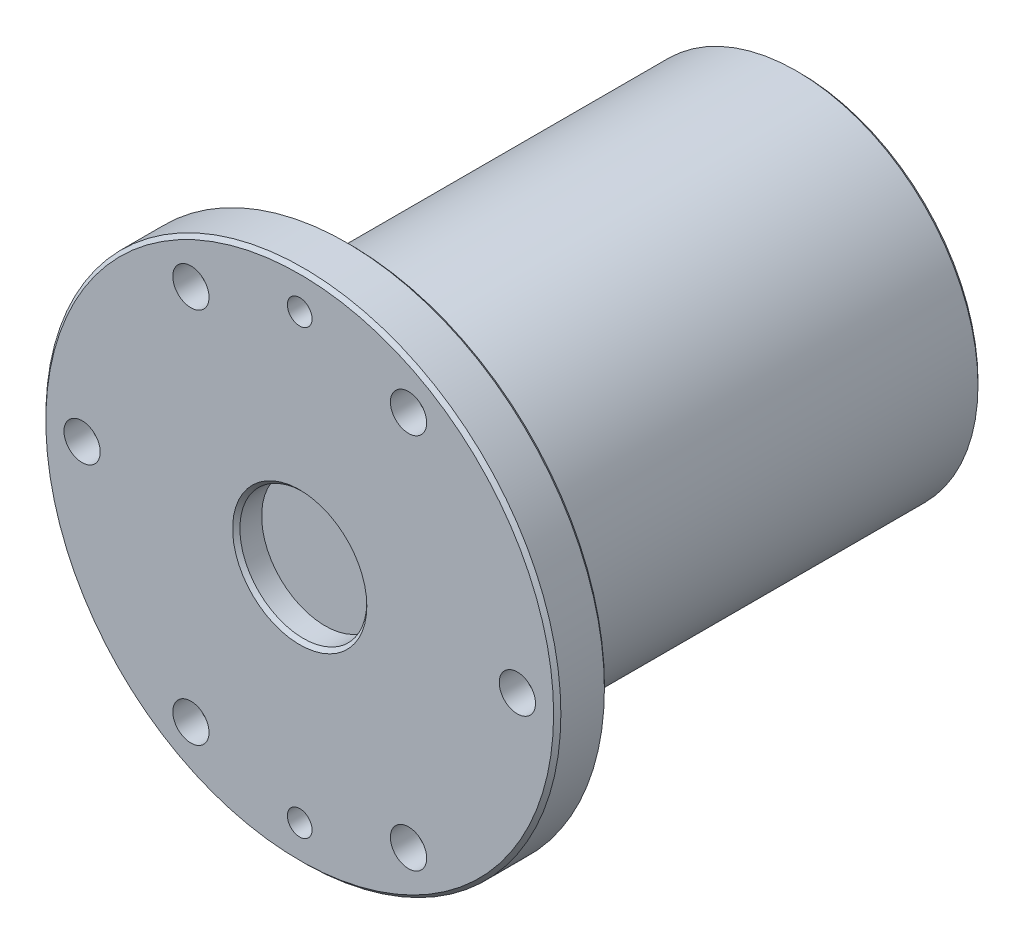
from build123d import *

# Parameters (mm, degrees)
SKETCH1_R           = 50
BOSS_EXTRUDE1_DEPTH = 138
BOSS_EXTRUDE2_START = -14
SKETCH6_R           = 71
SKETCH6_R_2         = 50
BOSS_EXTRUDE2_DEPTH = 14
CHAMFER3_SIZE       = 1
CHAMFER4_SIZE       = 1
CHAMFER5_SIZE       = 1
SKETCH7_R           = 17.5
CUT_EXTRUDE1_DEPTH  = 7
CHAMFER6_SIZE       = 1
CIRPATTERN1_COUNT   = 6
M8_TAPPED_HOLE1_D   = 6.8


with BuildPart() as part:
    # Sketch1 → Boss-Extrude1 (new body)
    with BuildSketch(Plane.XY):
        Circle(SKETCH1_R)
    extrude(amount=BOSS_EXTRUDE1_DEPTH)

    # Sketch6 → Boss-Extrude2 (add)
    with BuildSketch(Plane.XY.offset(138).offset(BOSS_EXTRUDE2_START)):
        Circle(SKETCH6_R)
        Circle(SKETCH6_R_2, mode=Mode.SUBTRACT)
    extrude(amount=BOSS_EXTRUDE2_DEPTH)

    # Chamfer3
    chamfer3_edges = [part.edges().sort_by_distance(p)[0] for p in [
        (-50, 0, 0),
    ]]
    chamfer(chamfer3_edges, length=CHAMFER3_SIZE)

    # Chamfer4
    chamfer4_edges = [part.edges().sort_by_distance(p)[0] for p in [
        (-71, 0, 138),
    ]]
    chamfer(chamfer4_edges, length=CHAMFER4_SIZE)

    # Chamfer5
    chamfer5_edges = [part.edges().sort_by_distance(p)[0] for p in [
        (-71, 0, 124),
    ]]
    chamfer(chamfer5_edges, length=CHAMFER5_SIZE)

    # Sketch7 → Cut-Extrude1 (cut)
    with BuildSketch(Plane.XY.offset(138)):
        Circle(SKETCH7_R)
    extrude(amount=-CUT_EXTRUDE1_DEPTH, mode=Mode.SUBTRACT)

    # Chamfer6
    chamfer6_edges = [part.edges().sort_by_distance(p)[0] for p in [
        (-17.5, 0, 138),
    ]]
    chamfer(chamfer6_edges, length=CHAMFER6_SIZE)

    # Sketch9 → Hole size (per socket head cap screw type)1 (revolve, cut)
    with BuildSketch(Plane(origin=(60, 0, 138), x_dir=(0, -1, 0), z_dir=(1, 0, 0))):
        Polygon((0, 0), (0, 15.652366702), (2.75, 14), (2.75, 7), (5, 7), (5, 0), align=None)
    hole_size_per_socket_head_cap_screw_typ = revolve(axis=Axis((60, 0, 144.35), (0, 0, -1)), mode=Mode.SUBTRACT)

    # CirPattern1: Hole size (per socket head cap screw type)1 ×6 about axis
    cirpattern1_axis = Axis((0, 0, 0), (0, 0, 1))
    for i in range(1, CIRPATTERN1_COUNT):
        add(hole_size_per_socket_head_cap_screw_typ.rotate(cirpattern1_axis, i * 360 / CIRPATTERN1_COUNT), mode=Mode.SUBTRACT)

    # M8 Tapped Hole1 (through all)
    with Locations(Plane.XY.offset(138)):
        with Locations((0, 61), (0, -61)):
            Hole(M8_TAPPED_HOLE1_D / 2)


solid = part.part
